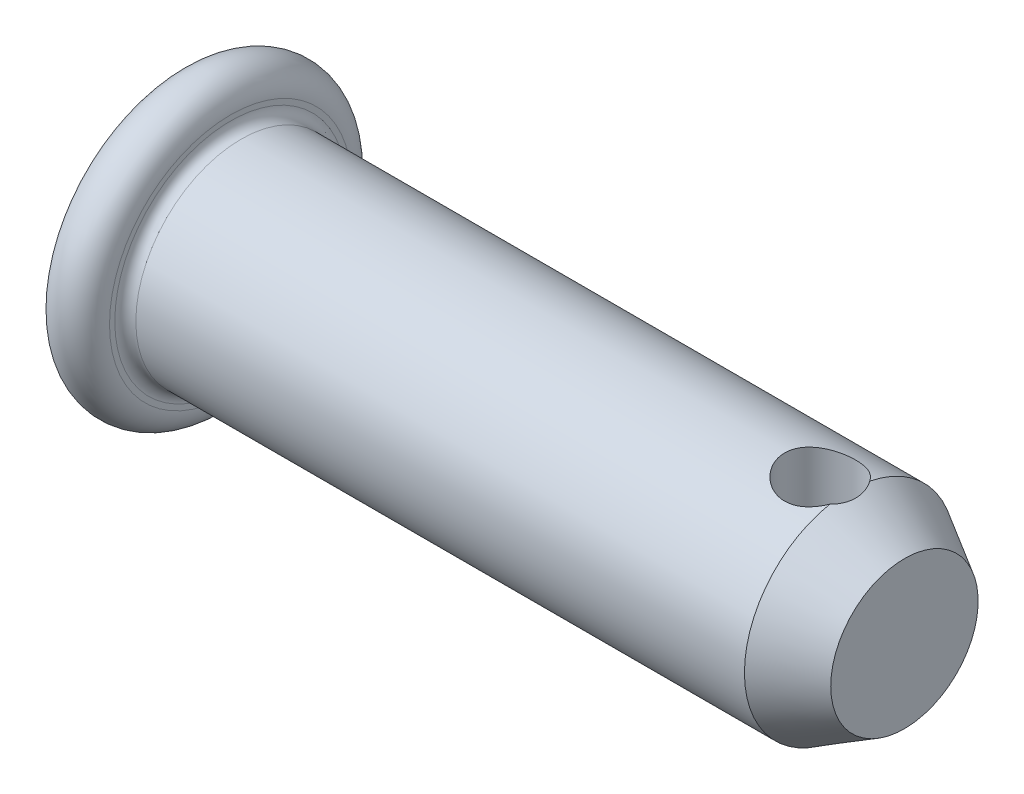
from build123d import *

# Parameters (mm, degrees)
FILLET_1_R          = 0.5
CHAMFER_1_SIZE      = 2.598076211
CHAMFER_1_SIZE2     = 1.5
SKETCH_2_R          = 1.69
CUT_EXTRUDE_1_DEPTH = 500


with BuildPart() as part:
    # 草图1 → Revolve 730 (revolve)
    with BuildSketch(Plane.XY, mode=Mode.PRIVATE) as revolve_730_sk:
        with BuildLine():
            Line((0, 0), (34.5, 0))
            Line((34.5, 0), (34.5, 5))
            Line((34.5, 5), (2.5, 5))
            Line((2.5, 5), (2.5, 5.75))
            ThreePointArc((2.5, 5.75), (1.25, 7), (0, 5.75))
            Line((0, 5.75), (0, 0))
        make_face()
    revolve(revolve_730_sk.sketch.rotate(Axis((0, 0, 0), (1, 0, 0)), 90), axis=Axis((0, 0, 0), (1, 0, 0)))

    # 圆角1
    fillet_1_edges = [part.edges().sort_by_distance(p)[0] for p in [
        (2.5, 0, -5),
    ]]
    fillet(fillet_1_edges, radius=FILLET_1_R)

    # 倒角1
    chamfer_1_edges = [part.edges().sort_by_distance(p)[0] for p in [
        (34.5, 0, -5),
    ]]
    chamfer_1_side = [part.faces().sort_by_distance(p)[0] for p in [
        (18.75, 0, -5),
    ]]
    chamfer(chamfer_1_edges, length=CHAMFER_1_SIZE, length2=CHAMFER_1_SIZE2, reference=chamfer_1_side[0])

    # 草图2 → 切除-拉伸1 (cut, symmetric)
    with BuildSketch(Plane(origin=(0, 0, 0), x_dir=(1, 0, 0), z_dir=(0, 1, 0))):
        with Locations(Location((30.5, 0, 0), (0, 0, 326.051586003))):
            Circle(SKETCH_2_R)
    extrude(amount=CUT_EXTRUDE_1_DEPTH, both=True, mode=Mode.SUBTRACT)


solid = part.part
